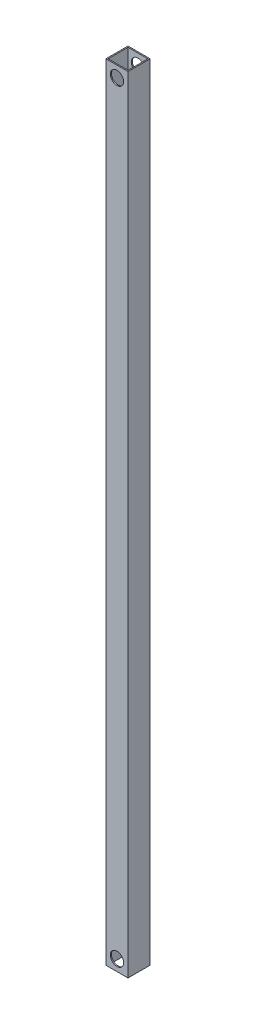
from build123d import *

# Parameters (mm, degrees)
SKETCH1_W           = 10
SKETCH1_H           = 10
SKETCH1_W_2         = 9
SKETCH1_H_2         = 9
BOSS_EXTRUDE1_DEPTH = 355
SKETCH2_R           = 3
CUT_EXTRUDE1_DEPTH  = 19
SKETCH3_R           = 3
CUT_EXTRUDE2_DEPTH  = 16


with BuildPart() as part:
    # Sketch1 → Boss-Extrude1 (new body)
    with BuildSketch(Plane(origin=(0, 0, 0), x_dir=(1, 0, 0), z_dir=(0, 1, 0))):
        Rectangle(SKETCH1_W, SKETCH1_H)
        Rectangle(SKETCH1_W_2, SKETCH1_H_2, mode=Mode.SUBTRACT)
    extrude(amount=BOSS_EXTRUDE1_DEPTH)

    # Sketch2 → Cut-Extrude1 (cut)
    with BuildSketch(Plane(origin=(0, 0, -5), x_dir=(-1, 0, 0), z_dir=(0, 0, -1))):
        with Locations((0, 5)):
            Circle(SKETCH2_R)
    extrude(amount=-CUT_EXTRUDE1_DEPTH, mode=Mode.SUBTRACT)

    # Sketch3 → Cut-Extrude2 (cut)
    with BuildSketch(Plane(origin=(0, 0, -5), x_dir=(-1, 0, 0), z_dir=(0, 0, -1))):
        with Locations((0, 350)):
            Circle(SKETCH3_R)
    extrude(amount=-CUT_EXTRUDE2_DEPTH, mode=Mode.SUBTRACT)


solid = part.part
